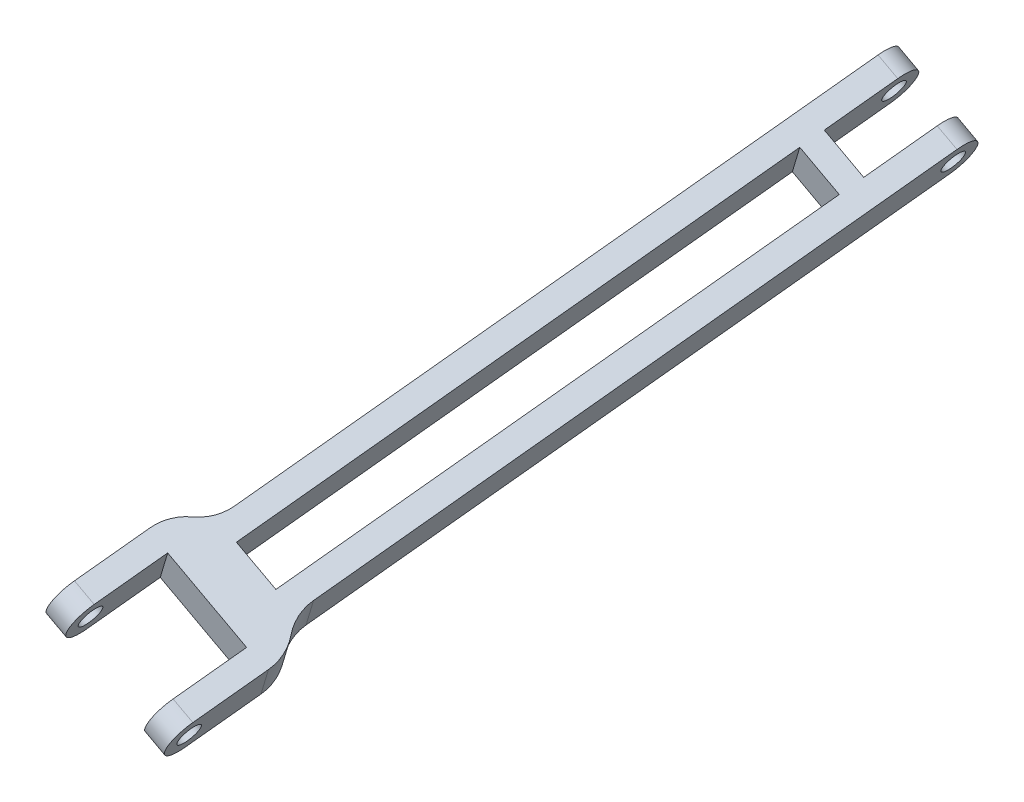
SolidWorks part; units mm, degrees
ref_plane "Front Plane" through (0, 0, 0) normal (0, 0, 1) x (1, 0, 0)
ref_plane "Top Plane" through (0, 0, 0) normal (0, 1, 0) x (1, 0, 0)
ref_plane "Right Plane" through (0, 0, 0) normal (1, 0, 0) x (0, 0, -1)
ref_plane "Plane4" through (5.22, -2.8042, 0) normal (-0.8809, 0.4732, 0) x (-0.4732, -0.8809, 0)
sketch "Sketch1" plane through (5.22, -2.8042, 0) normal (-0.8809, 0.4732, 0) x (-0.4732, -0.8809, 0)
  line L0 (88.7142, -264.6258) -> (65.7331, -341.254)
  line L1 (70.5224, -342.6903) -> (93.5034, -266.0621)
  arc A0 (65.7331, -341.254) -> (70.5224, -342.6903) centre (68.1277, -341.9721) ccw
  arc A1 (93.5034, -266.0621) -> (88.7142, -264.6258) centre (91.1088, -265.344) ccw
extrude "Boss-Extrude1" add sketch "Sketch1" against normal blind 15
sketch "Sketch2" plane through (-75.2427, -140.0652, -47.6835) normal (-0.4533, -0.8438, -0.2873) x (0.8914, -0.4291, -0.1461)
  line L0 (57.7695, -302.7188) -> (62.711, -301.9562)
  line L1 (62.711, -301.9562) -> (61.5671, -294.5439)
  line L2 (61.5671, -294.5439) -> (56.6256, -295.3065)
  line L3 (56.6256, -295.3065) -> (57.7695, -302.7188)
extrude "Cut-Extrude1" cut sketch "Sketch2" against normal through all
sketch "Sketch3" plane through (-75.2427, -140.0652, -47.6835) normal (-0.4533, -0.8438, -0.2873) x (0.8914, -0.4291, -0.1461)
  line L0 (41.8038, -232.0427) -> (52.828, -303.4813)
  line L1 (52.828, -303.4813) -> (55.2987, -303.1)
  line L2 (55.2987, -303.1) -> (45.2833, -238.1984)
  arc A0 (45.2833, -238.1984) -> (43.5435, -235.1205) centre (40.3418, -238.9609) ccw
  arc A1 (43.5435, -235.1205) -> (41.8038, -232.0427) centre (46.7453, -231.2801) cw
extrude "Cut-Extrude2" cut sketch "Sketch3" against normal through all
sketch "Sketch4" plane through (-75.2427, -140.0652, -47.6835) normal (-0.4533, -0.8438, -0.2873) x (0.8914, -0.4291, -0.1461)
  line L0 (43.0978, -224.0359) -> (44.2416, -231.4482)
  line L1 (44.2416, -231.4482) -> (54.1246, -229.923)
  line L2 (54.1246, -229.923) -> (52.9808, -222.5108)
  line L3 (52.9808, -222.5108) -> (43.0978, -224.0359)
extrude "Cut-Extrude3" cut sketch "Sketch4" against normal through all
sketch "Sketch5" plane through (-75.2427, -140.0652, -47.6835) normal (-0.4533, -0.8438, -0.2873) x (0.8914, -0.4291, -0.1461)
  line L0 (67.6525, -301.1936) -> (56.6283, -229.755)
  line L1 (55.1663, -236.6733) -> (65.1817, -301.5749)
  line L2 (65.1817, -301.5749) -> (67.6525, -301.1936)
  arc A0 (56.6283, -229.755) -> (55.8973, -233.2141) centre (51.6868, -230.5175) cw
  arc A1 (55.8973, -233.2141) -> (55.1663, -236.6733) centre (60.1078, -235.9107) ccw
extrude "Cut-Extrude4" cut sketch "Sketch5" against normal through all
sketch "Sketch6" plane through (-75.2427, -140.0652, -47.6835) normal (-0.4533, -0.8438, -0.2873) x (0.8914, -0.4291, -0.1461)
  line L0 (56.2444, -292.8357) -> (61.1859, -292.0732)
  line L1 (61.1859, -292.0732) -> (52.4164, -235.2458)
  line L2 (52.4164, -235.2458) -> (47.4749, -236.0084)
  line L3 (47.4749, -236.0084) -> (56.2444, -292.8357)
extrude "Cut-Extrude5" cut sketch "Sketch6" against normal through all
hole_wizard "Ø2.5 (2.5) Diameter Hole1" positions "Sketch8" profile "Sketch7" hole size "Ø2.5" standard "ANSI Metric"
sketch "Sketch8" plane through (16.2317, -8.7196, 0) normal (0.8809, -0.4732, 0) x (0, 0, -1)
  point P0 (341.9721, -68.1277)
sketch "Sketch7" plane through (-16.0088, -68.7358, -341.9721) normal (0, 0, 1) x (0.4732, 0.8809, 0)
  line L0 (0, 0) -> (0, 2.5)
  line L1 (0, 2.5) -> (1.25, 2.5)
  line L2 (1.25, 2.5) -> (1.25, 0)
  line L5 (1.25, 0) -> (0, 0)
  line L11 (0, -6.35) -> (0, 107.95) construction
  dimension "通孔孔直径" = 2.5
  dimension "通孔孔深度" = 2.5
hole_wizard "Ø2.5 (2.5) Diameter Hole2" positions "Sketch10" profile "Sketch9" hole size "Ø2.5" standard "ANSI Metric"
sketch "Sketch10" plane through (9.6247, -5.1703, 0) normal (0.8809, -0.4732, 0) x (0, 0, -1)
  point P0 (341.9721, -68.1277)
sketch "Sketch9" plane through (-22.6159, -65.1865, -341.9721) normal (0, 0, 1) x (0.4732, 0.8809, 0)
  line L0 (0, 0) -> (0, 2.5)
  line L1 (0, 2.5) -> (1.25, 2.5)
  line L2 (1.25, 2.5) -> (1.25, 0)
  line L5 (1.25, 0) -> (0, 0)
  line L11 (0, -6.35) -> (0, 107.95) construction
  dimension "通孔孔直径" = 2.5
  dimension "通孔孔深度" = 2.5
hole_wizard "Ø2.5 (2.5) Diameter Hole3" positions "Sketch12" profile "Sketch11" hole size "Ø2.5" standard "ANSI Metric"
sketch "Sketch12" plane through (18.434, -9.9027, 0) normal (0.8809, -0.4732, 0) x (0, 0, -1)
  point P0 (265.344, -91.1088)
sketch "Sketch11" plane through (-24.682, -90.1637, -265.344) normal (0, 0, 1) x (0.4732, 0.8809, 0)
  line L0 (0, 0) -> (0, 2.5)
  line L1 (0, 2.5) -> (1.25, 2.5)
  line L2 (1.25, 2.5) -> (1.25, 0)
  line L5 (1.25, 0) -> (0, 0)
  line L11 (0, -6.35) -> (0, 107.95) construction
  dimension "通孔孔直径" = 2.5
  dimension "通孔孔深度" = 2.5
hole_wizard "Ø2.5 (2.5) Diameter Hole4" positions "Sketch14" profile "Sketch13" hole size "Ø2.5" standard "ANSI Metric"
sketch "Sketch14" plane through (7.4223, -3.9872, 0) normal (0.8809, -0.4732, 0) x (0, 0, -1)
  point P0 (265.344, -91.1088)
sketch "Sketch13" plane through (-35.6937, -84.2482, -265.344) normal (0, 0, 1) x (0.4732, 0.8809, 0)
  line L0 (0, 0) -> (0, 14.165)
  line L1 (0, 14.165) -> (1.25, 14.165)
  line L2 (1.25, 14.165) -> (1.25, 0)
  line L5 (1.25, 0) -> (0, 0)
  line L11 (0, -6.35) -> (0, 107.95) construction
  dimension "通孔孔直径" = 2.5
  dimension "通孔孔深度" = 14.165
sketch "Sketch16" plane through (-75.2427, -140.0652, -47.6835) normal (-0.4533, -0.8438, -0.2873) x (0.8914, -0.4291, -0.1461)
  line L0 (43.0978, -224.0359) -> (42.7165, -221.5651)
  line L1 (55.0703, -219.6587) -> (40.2457, -221.9464) construction
  line L2 (42.7165, -221.5651) -> (52.5995, -220.04)
  line L3 (52.5995, -220.04) -> (52.9808, -222.5108)
  line L4 (40.4364, -223.1818) -> (40.8177, -225.6526) construction
  line L5 (55.4515, -222.1295) -> (55.0703, -219.6587) construction
  line L6 (43.0978, -224.0359) -> (52.9808, -222.5108)
extrude "Cut-Extrude6" cut sketch "Sketch16" against normal blind 10
sketch "Sketch17" plane through (-75.2427, -140.0652, -47.6835) normal (-0.4533, -0.8438, -0.2873) x (0.8914, -0.4291, -0.1461)
  line L1 (65.1817, -301.5749) -> (65.563, -304.0457)
  line L2 (53.2092, -305.9521) -> (68.0338, -303.6644) construction
  line L4 (55.68, -305.5708) -> (55.2987, -303.1)
  line L5 (55.2987, -303.1) -> (52.828, -303.4813)
  line L7 (52.828, -303.4813) -> (53.2092, -305.9521)
  line L8 (53.2092, -305.9521) -> (55.68, -305.5708)
  line L9 (65.1817, -301.5749) -> (67.6525, -301.1936)
  line L10 (67.6525, -301.1936) -> (68.0338, -303.6644)
  line L11 (68.0338, -303.6644) -> (65.563, -304.0457)
  line L12 (57.7695, -302.7188) -> (62.711, -301.9562)
  line L13 (62.711, -301.9562) -> (63.0923, -304.4269)
  line L14 (63.0923, -304.4269) -> (58.1507, -305.1895)
  line L15 (58.1507, -305.1895) -> (57.7695, -302.7188)
extrude "Cut-Extrude7" cut sketch "Sketch17" against normal blind 10
